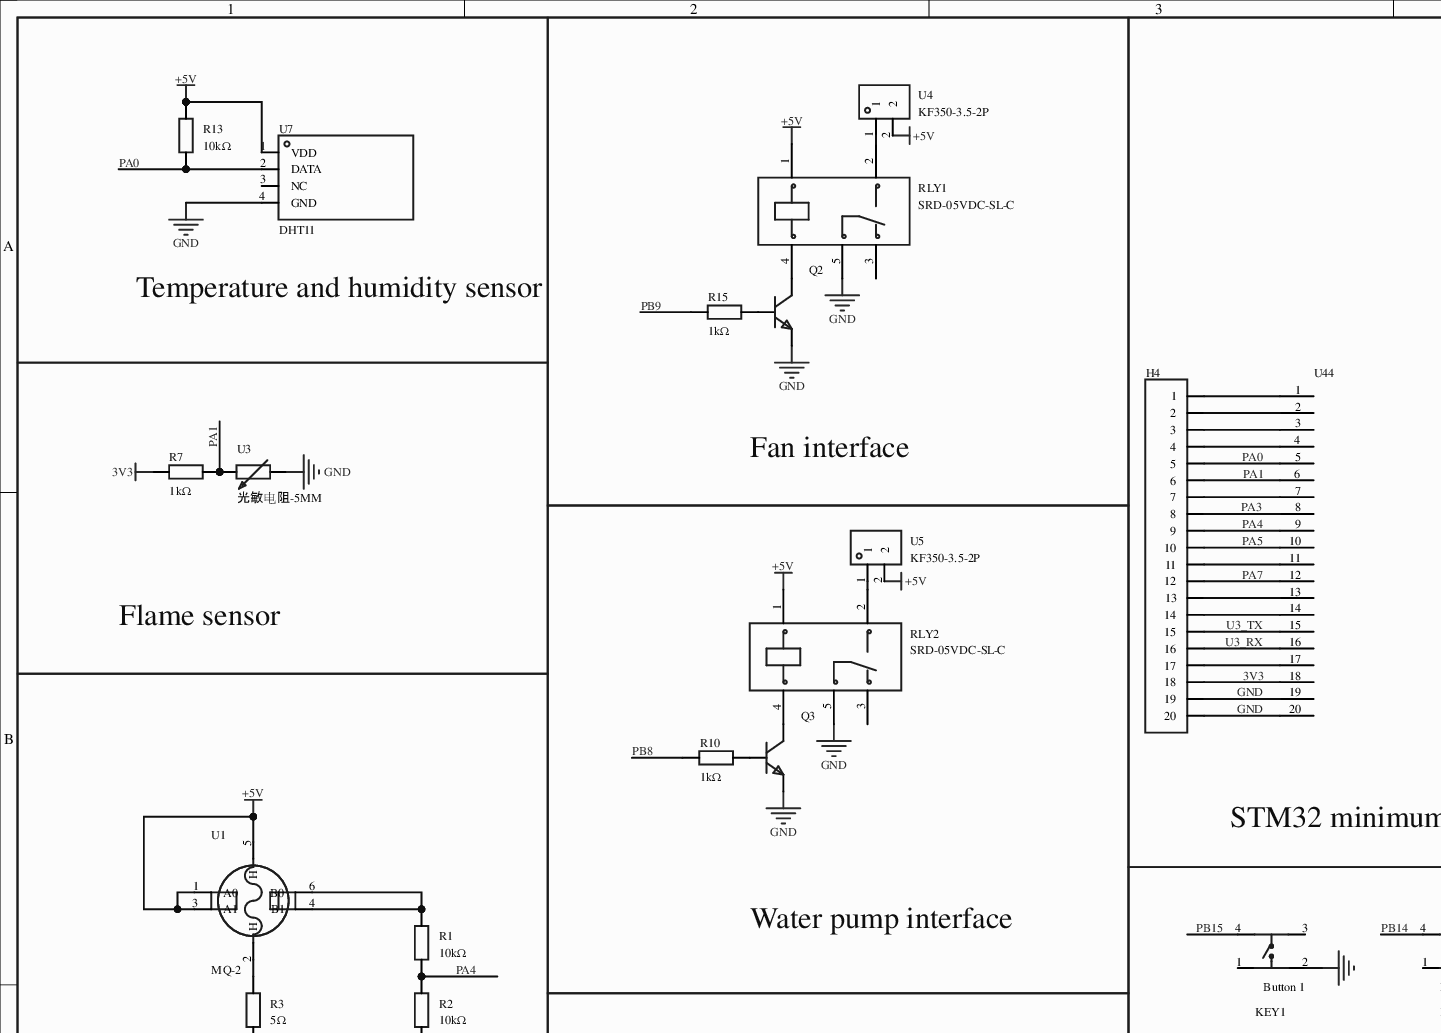
[diagram p0: MISC62290-3.schdoc, top left]
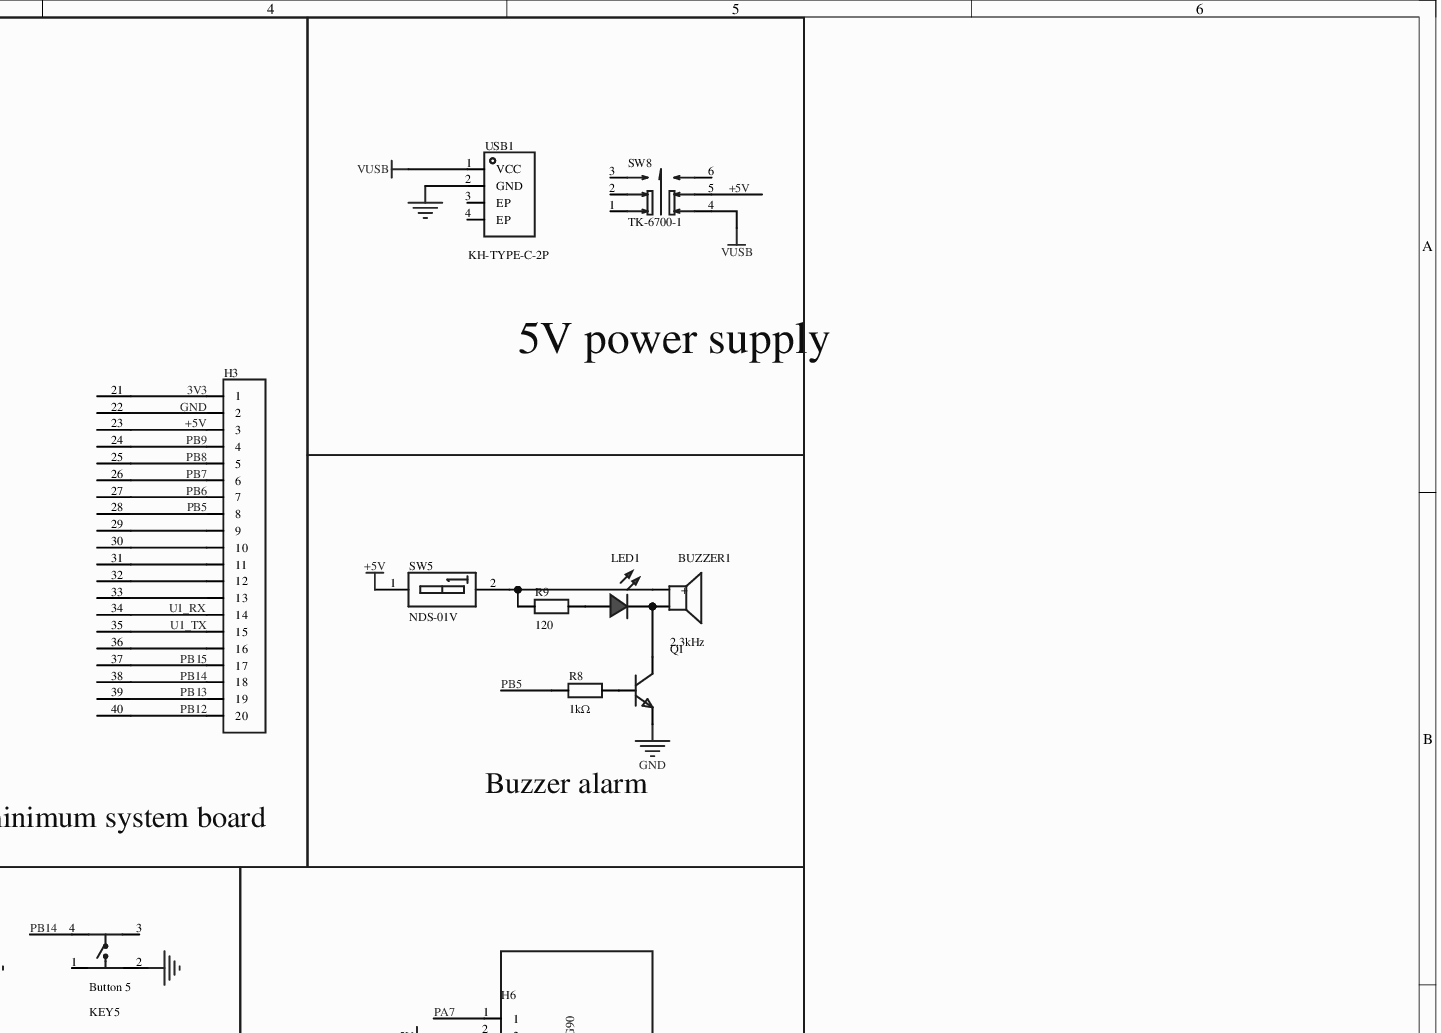
[diagram p1: MISC62290-3.schdoc, top right]
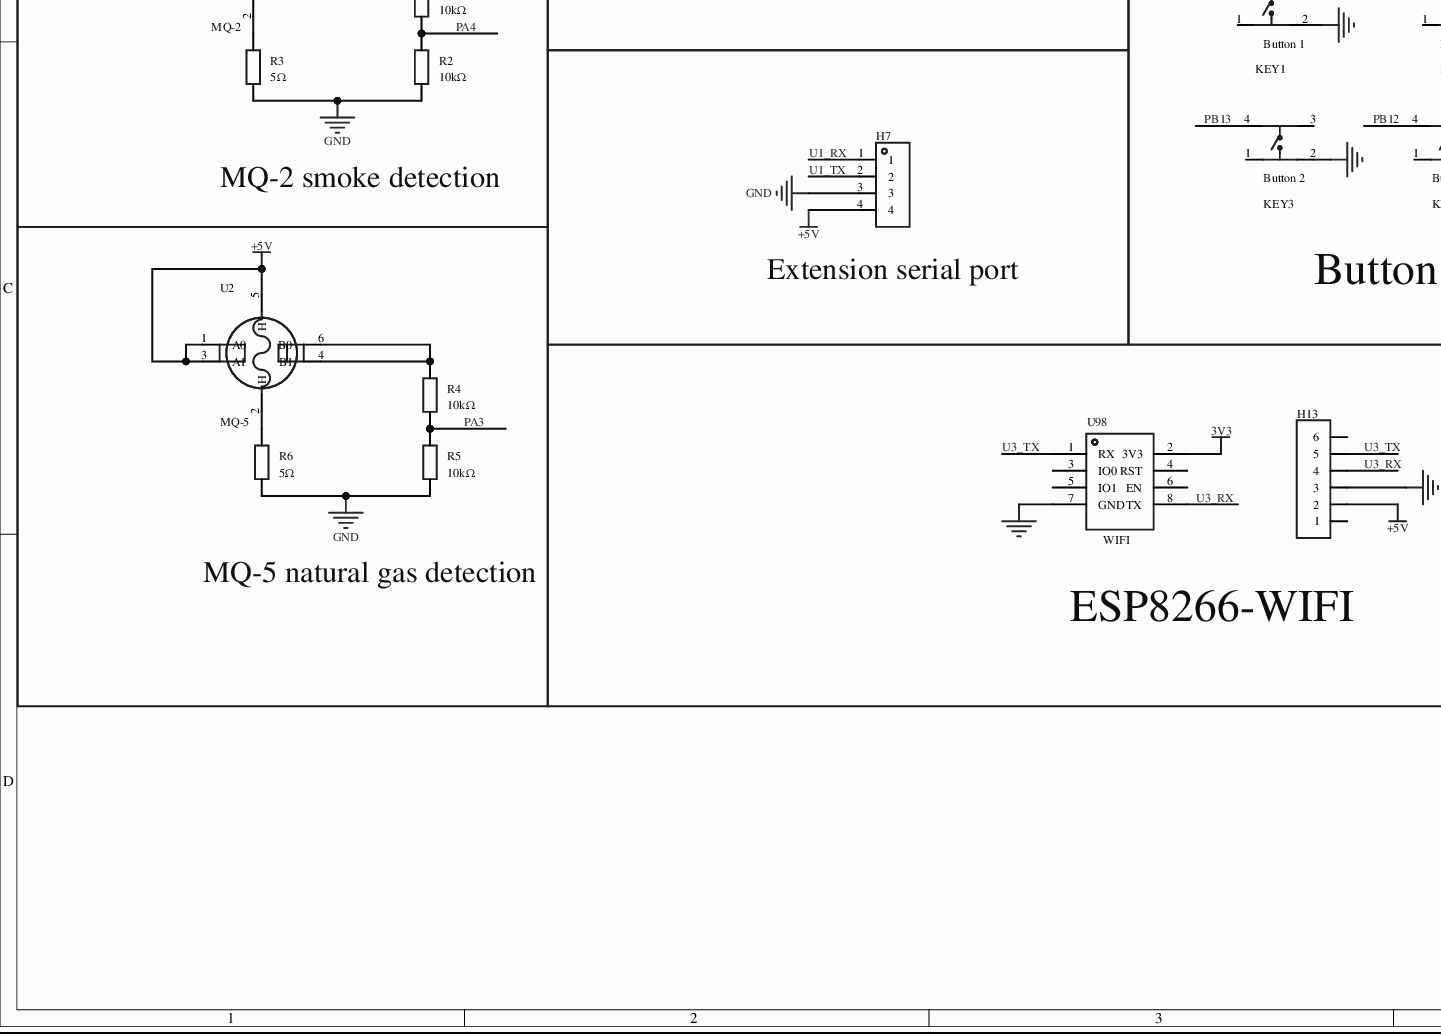
[diagram p2: MISC62290-3.schdoc, bottom left]
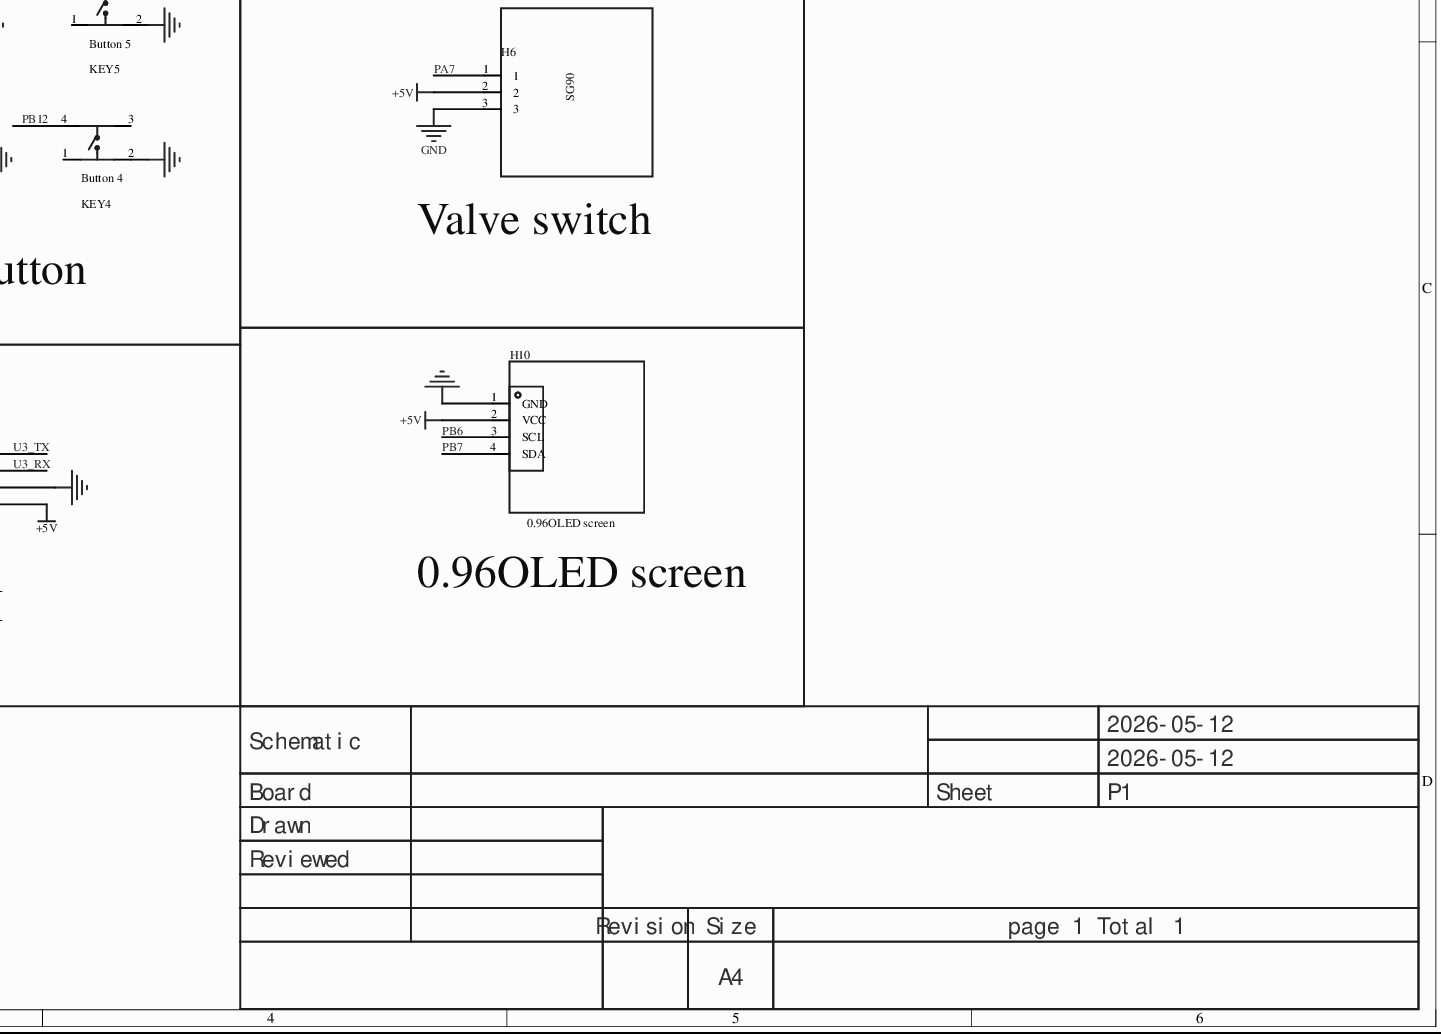
[diagram p3: MISC62290-3.schdoc, bottom right]
# Altium project MISC62290-2.PrjPcb
1 sheet, 40 parts. Net scope: global (net labels, ports and power ports of the same name join across sheets).
Board file: MISC62290.pcbdoc

## Sheet MISC62290-3.schdoc
size 420 x 297 mm; Version: V1.0; @Project Name: MISC62290; @Update Date: 2026-05-12; @Create Date: 2026-05-12; @Board Name: MISC62290; @Create Time: 10:51:37; @Page Count: 1; @Page No: 1; @Schematic Name: MISC62290; @Update Time: 10:51:37; Size: A4

### Parts
BUZZER1  2.3kHz  [BUZ-TH_BD12.0-P7.60-D0.6-FD]
H3  (no value)  [HDR-TH_20P-P2.54-V-F]
H4  (no value)  [HDR-TH_20P-P2.54-V-F]
H6  (no value)  [HDR-TH_3P-P2.54-V-F]
H7  (no value)  [HDR-TH_4P-P2.54-V-F]
H10  2.54-1*4P female  [HDR-TH_4P-P2.54-V-F]  (value not drawn)
H13  (no value)  [HDR-TH_6P-P2.54-V-M-1]
KEY1  Button 1  [KEY-TH_4P-L6.0-W6.0-P4.50-LS7.5]
KEY3  Button 2  [KEY-TH_4P-L6.0-W6.0-P4.50-LS7.5]
KEY4  Button 4  [KEY-TH_4P-L6.0-W6.0-P4.50-LS7.5]
KEY5  Button 5  [KEY-TH_4P-L6.0-W6.0-P4.50-LS7.5]
LED1  (no value)  [LED_TH-3mm]
Q1  (no value)  [S8050_TO_92]
Q2  (no value)  [S8050_TO_92]
Q3  (no value)  [S8050_TO_92]
R1  10kΩ  [Res_1/4W]
R2  10kΩ  [Res_1/4W]
R3  5Ω  [Res_1/4W]
R4  10kΩ  [Res_1/4W]
R5  10kΩ  [Res_1/4W]
R6  5Ω  [Res_1/4W]
R7  1kΩ  [Res_1/4W]
R8  1kΩ  [Res_1/4W]
R9  120  [Res_1/4W]
R10  1kΩ  [Res_1/4W]
R13  10kΩ  [Res_1/4W]
R15  1kΩ  [Res_1/4W]
RLY1  SRD-05VDC-SL-C  [RELAY-TH_SRD-XXVDC-XL-C]
RLY2  SRD-05VDC-SL-C  [RELAY-TH_SRD-XXVDC-XL-C]
SW5  NDS-01V  [SW-TH_2P-L3.9-W9.9-P2.54-LS7.6]
SW8  TK-6700-1  [SW-TH_TK-6700-1]
U1  MQ-2  [SENSOR-TH_MQ-2]
U2  MQ-5  [SENSOR-TH_MQ-2]
U3  光敏电阻-5MM  [RES-TH_L4.9-W4.3-P3.4]
U4  KF350-3.5-2P  [CONN-TH_P3.50_KF350-3.5-2P]
U5  KF350-3.5-2P  [CONN-TH_P3.50_KF350-3.5-2P]
U7  DHT11  [SENSOR-TH_DHT11]
U44  (no value)  [STM32最小系统板]
U98  (no value)  [WiFi封装]
USB1  KH-TYPE-C-2P  [USB-SMD_KH-TYPE-C-2P]

### Blocks framed on the sheet
Temperature and humidity sensor: R13 U7
Fan interface: Q2 R15 RLY1 U4
STM32 minimum system board: H3 H4 U44
5V power supply: SW8 USB1
Flame sensor: R7 U3
Buzzer alarm: BUZZER1 LED1 Q1 R8 R9 SW5
Water pump interface: Q3 R10 RLY2 U5
MQ-2 smoke detection: R1-R3 U1
Button: KEY1 KEY3-KEY5
Valve switch: H6
Extension serial port: H7
MQ-5 natural gas detection: R4-R6 U2
ESP8266-WIFI: H13 U98
0.96OLED screen: H10

### Nets
3V3: H3.1 H4.18 R7.1 U44.18 U44.21 U98.2(3V3)
+5V: H3.3 H6.2 H7.4 H10.2(VCC) H13.2 R13.2 RLY1.1 RLY2.1 SW5.1(A1) SW8.5 U1.1(A0) U1.3(A1) U1.5(H) U2.1(A0) U2.3(A1) U2.5(H) U4.2 U5.2 U7.1(VDD) U44.23
GND: H3.2 H4.19 H4.20 H6.3 H7.3 H10.1(GND) H13.3 KEY1.2 KEY3.2 KEY4.2 KEY5.2 Q1.1(E) Q2.1(E) Q3.1(E) R2.1 R3.1 R5.1 R6.1 RLY1.5 RLY2.5 U3.1 U7.4(GND) U44.19 U44.20 U44.22 U98.7(GND) USB1.2(GND)
VUSB: SW8.4 USB1.1(VCC)
PA0: H4.5 R13.1 U7.2(DATA) U44.5
PA1: H4.6 R7.2 U3.2 U44.6
PA3: H4.8 R4.1 R5.2 U44.8
PA4: H4.9 R1.1 R2.2 U44.9
PA5: H4.10 U44.10
PA7: H4.12 H6.1 U44.12
PB5: H3.8 R8.1 U44.28
PB6: H3.7 H10.3(SCL) U44.27
PB7: H3.6 H10.4(SDA) U44.26
PB8: H3.5 R10.1 U44.25
PB9: H3.4 R15.1 U44.24
PB12: H3.20 KEY4.4 U44.40
PB13: H3.19 KEY3.4 U44.39
PB14: H3.18 KEY5.4 U44.38
PB15: H3.17 KEY1.4 U44.37
U1_RX: H3.14 H7.1 U44.34
U1_TX: H3.15 H7.2 U44.35
U3_RX: H4.16 H13.4 U44.16 U98.8(TX)
U3_TX: H4.15 H13.5 U44.15 U98.1(RX)
NetBUZZER1_1: BUZZER1.1(+) R9.1 SW5.2(A2)
NetBUZZER1_2: BUZZER1.2 LED1.2(A) Q1.3(C)
NetH3_9: H3.9 U44.29
NetH3_10: H3.10 U44.30
NetH3_11: H3.11 U44.31
NetH3_12: H3.12 U44.32
NetH3_13: H3.13 U44.33
NetH3_16: H3.16 U44.36
NetH4_1: H4.1 U44.1
NetH4_2: H4.2 U44.2
NetH4_3: H4.3 U44.3
NetH4_4: H4.4 U44.4
NetH4_7: H4.7 U44.7
NetH4_11: H4.11 U44.11
NetH4_13: H4.13 U44.13
NetH4_14: H4.14 U44.14
NetH4_17: H4.17 U44.17
NetLED1_1: LED1.1(C) R9.2
NetQ1_2: Q1.2(B) R8.2
NetQ2_2: Q2.2(B) R15.2
NetQ2_3: Q2.3(C) RLY1.4
NetQ3_2: Q3.2(B) R10.2
NetQ3_3: Q3.3(C) RLY2.4
NetR1_2: R1.2 U1.4(B1) U1.6(B0)
NetR3_2: R3.2 U1.2(H)
NetR4_2: R4.2 U2.4(B1) U2.6(B0)
NetR6_2: R6.2 U2.2(H)
NetRLY1_2: RLY1.2 U4.1
NetRLY2_2: RLY2.2 U5.1

Not connected (* = marked no-connect by the designer): H13 1 6; KEY1 1 3*; KEY3 1 3*; KEY4 1 3*; KEY5 1 3*; RLY1 3; RLY2 3; SW8 1* 2* 3* 6*; U7 3(NC); U98 3(IO0) 4(RST) 5(IO1) 6(EN); USB1 3(EP) 4(EP)

### Notes on the sheet
- 2026-05-12
- Schematic
- Board
- Sheet
- P1
- Drawn
- Reviewed
- Revision
- Size
- A4
- page 1 Total 1

### Library data of the parts
BUZZER1 = TMB12A05_C96093: Drive method: active (built-in driver circuit); Construction type: electromagnetic; Rated voltage: 5V; Frequency: 2.3kHz; Sound pressure (SPL): 85dB@5V,10cm;; Manufacturer: 华能; 3D Model: 16ab50e14c5b4f2c986c135bdba60e37; 3D Model Transform: 472.44,472.176,0,90,0,0,-0.787,0,-177.165; Oscillator Circuit: Active (built-in driver); Operating Voltage: 4V~8V; AddInBom: yes; ModelName: BUZ-TH_D12.0-H9.5-P7.60; Symbol: TMB12A05; Device: TMB12A05_C96093; LCSC Part Name: TMB12A05; Supplier Part: C96093; Manufacturer Part: TMB12A05; Supplier Footprint: 插件,D=12mm; JLCPCB Part Class: Extended Part; Datasheet: https://atta.szlcsc.com/upload/public/pdf/source/20170522/1495448324811.pdf; Supplier: LCSC; Technology Type: Electromagnetic; Rated Voltage: 5V; Value: 2.3kHz; Sound Pressure Level (SPL): 85dB@5V,10cm; Diameter (φD): 12mm; Height: 9.8mm; ConvertToPcb: yes; FootprintName: BUZ-TH_BD12.0-P7.60-D0.6-FD
H3 H4 = HDR-F_2.54_1x20P: ConvertToPcb: yes; ModelId: db7015f7ad9d48b8a3b1188db02e34290819f05c4eef4c71ace90d822a990e87; ModelName: HDR-F-2.54_1x20; ModelTransform: 1999.996,100,0,0,0,0,0,0,-118.11; Symbol: HDR-F_2.54_1x20P; Device: HDR-F_2.54_1x20P; AddInBom: yes; SupplierPart: C50984; Supplier Footprint: 插件; FootprintName: HDR-TH_20P-P2.54-V-F
H6 = HDR-F_2.54_1x3P: Symbol: PM254V-11-03-H85_1; 3D Model: f3b3cc5aae9641bf9e56fc160cef875b; 3D Model Transform: 299.9994,100,0,0,0,0,0,0,-118.11; ConvertToPcb: yes; ModelName: HDR2.54-F-LI-1X3P; Device: HDR-F_2.54_1x3P; Supplier Part: C541850; Supplier Footprint: 插件; AddInBom: yes; FootprintName: HDR-TH_3P-P2.54-V-F
H7 = HDR-F_2.54_1x4P: Symbol: 2.54-1*4P female; ConvertToPcb: yes; ModelId: d187812051054f85879fcaa51a310d8e0819f05c4eef4c71ace90d822a990e87; ModelTransform: 419.6842,98.464,0,0,0,0,0,0,-118.11; Device: HDR-F_2.54_1x4P; AddInBom: yes; SupplierPart: C2718488; Supplier Footprint: 插件; FootprintName: HDR-TH_4P-P2.54-V-F; ModelName: HDR-TH_4P-P2.54-V-F
H10 = 0.96OLED屏幕: Socket structure: 1x4P; Pitch: 2.54mm; Row spacing: -; Round/square hole: square hole; Mounting type: through-hole; Rows: single row; Total positions: 4P; Rated current: 3A; Rated voltage: -; Socket direction: top; Plastic height: -; Contact material: bronze; Contact plating: -; Operating temperature range: -40℃~+105℃; Soldering temperature (max): -;; Manufacturer: BOOMELE(博穆精密); Manufacturer Part: 2.54-1*4P母; Symbol: 0.96OLED screen; 3D Model: 57daaad411c24bd7bd5d06edf5c4d16b; 3D Model Transform: 415.7472,98.425,0,0,0,0,0,0,-118.11; AddInBom: yes; ModelName: HDR-TH_4P-P2.54-F-LI-1X4P; Device: 0.96OLED screen; Supplier: LCSC; Supplier Part: C2718488; JLCPCB Part Class: Extension library; LCSC Part Name: 间距:2.54mm 1x4P 直插; Supplier Footprint: 插件,P=2.54mm; Datasheet: https://atta.szlcsc.com/upload/public/pdf/source/20210301/C2718488_F4427B881E42CAA8DDB0B1C12B3A522C.pdf; Holes Structure: 1x4P; Row Spacing: -; Circular Hole / Square Hole: Square hole; Mounting Type: Through-hole; Number of Rows: Single row; Number of Holes: 4P; Current Rating (Max): 3A; Voltage Rating (Max): -; Holes Direction: Top; Insulation Height: -; Contact Material: Bronze; Contact Plating: -; Operating Temperature Range: -40℃~+105℃; Soldering Temperature(Max): -; ConvertToPcb: yes; FootprintName: HDR-TH_4P-P2.54-V-F
H13 = HDR-M_2.54_1x6P: Symbol: Header-Male-2.54_1x6; 3D Model: 60739dffc9b04830a286435b0fefbd4a; 3D Model Transform: 599.999,100,0,0,0,0,0,0,-118.11; ConvertToPcb: yes; ModelName: HDR2.54-M-LI-1X6P; Device: HDR-M_2.54_1x6P; Supplier Part: C37208; Supplier Footprint: 插件; AddInBom: yes; FootprintName: HDR-TH_6P-P2.54-V-M-1
KEY1 = 按键开关6*6*8: Circuit structure: SPST; Contact rated current: -; Button head type: Round Button; Button actuation direction: Top Actuated;; Manufacturer Part: 按键1; Symbol: button6*6*8; Device: Tact switch 6*6*8; 3D Model: 84d39232fe0a426fa95ea2653754a6e5; 3D Model Transform: 306.868,236.22,0,0,0,0,0,0,-118.11; AddInBom: yes; ModelName: KEY-TH_4P-L6.0-W6.0-H4.5-LS6.5-P4.5; LCSC Part Name: 按键开关6*6*8   直插; Supplier Part: C59982; Supplier Footprint: Through Hole; JLCPCB Part Class: Extension library; Datasheet: https://atta.szlcsc.com/upload/public/pdf/source/20151126/1457707591845.pdf; Supplier: LCSC; ConvertToPcb: yes; FootprintName: KEY-TH_4P-L6.0-W6.0-P4.50-LS7.5
KEY3 = 按键开关6*6*8: Circuit structure: SPST; Contact rated current: -; Button head type: Round Button; Button actuation direction: Top Actuated;; Manufacturer Part: 按键2; Symbol: button6*6*8; Device: Tact switch 6*6*8; 3D Model: 84d39232fe0a426fa95ea2653754a6e5; 3D Model Transform: 306.868,236.22,0,0,0,0,0,0,-118.11; AddInBom: yes; ModelName: KEY-TH_4P-L6.0-W6.0-H4.5-LS6.5-P4.5; LCSC Part Name: 按键开关6*6*8   直插; Supplier Part: C59982; Supplier Footprint: Through Hole; JLCPCB Part Class: Extension library; Datasheet: https://atta.szlcsc.com/upload/public/pdf/source/20151126/1457707591845.pdf; Supplier: LCSC; ConvertToPcb: yes; FootprintName: KEY-TH_4P-L6.0-W6.0-P4.50-LS7.5
KEY4 = 按键开关6*6*8: Circuit structure: SPST; Contact rated current: -; Button head type: Round Button; Button actuation direction: Top Actuated;; Manufacturer Part: 按键4; Symbol: button6*6*8; Device: Tact switch 6*6*8; 3D Model: 84d39232fe0a426fa95ea2653754a6e5; 3D Model Transform: 306.868,236.22,0,0,0,0,0,0,-118.11; AddInBom: yes; ModelName: KEY-TH_4P-L6.0-W6.0-H4.5-LS6.5-P4.5; LCSC Part Name: 按键开关6*6*8   直插; Supplier Part: C59982; Supplier Footprint: Through Hole; JLCPCB Part Class: Extension library; Datasheet: https://atta.szlcsc.com/upload/public/pdf/source/20151126/1457707591845.pdf; Supplier: LCSC; ConvertToPcb: yes; FootprintName: KEY-TH_4P-L6.0-W6.0-P4.50-LS7.5
KEY5 = 按键开关6*6*8: Circuit structure: SPST; Contact rated current: -; Button head type: Round Button; Button actuation direction: Top Actuated;; Manufacturer Part: 按键5; Symbol: button6*6*8; Device: Tact switch 6*6*8; 3D Model: 84d39232fe0a426fa95ea2653754a6e5; 3D Model Transform: 306.868,236.22,0,0,0,0,0,0,-118.11; AddInBom: yes; ModelName: KEY-TH_4P-L6.0-W6.0-H4.5-LS6.5-P4.5; LCSC Part Name: 按键开关6*6*8   直插; Supplier Part: C59982; Supplier Footprint: Through Hole; JLCPCB Part Class: Extension library; Datasheet: https://atta.szlcsc.com/upload/public/pdf/source/20151126/1457707591845.pdf; Supplier: LCSC; ConvertToPcb: yes; FootprintName: KEY-TH_4P-L6.0-W6.0-P4.50-LS7.5
LED1 = LED_TH-R_3mm: ConvertToPcb: yes; ModelId: a497c992633541038a38947cdc58012f0819f05c4eef4c71ace90d822a990e87; ModelName: LED-TH-3mm_R; ModelTransform: 141.274,153.327,0,0,0,0,-5.984,0,-137.795; Symbol: LED_TH-R; Device: LED_TH-R_3mm; AddInBom: yes; FootprintName: LED_TH-3mm; Supplier Footprint: 插件
Q1-Q3 = S8050_TO_NPN: 3D Model: aafe8e06f2154e7c93506efd0d6632dd; 3D Model Transform: 180.78,141.44,417.3,0,0,0,0,0,-200; ConvertToPcb: yes; ModelName: TO-92-3_L4.9-W3.7-P1.27-L; Symbol: S8050_TO_NPN; Device: S8050_TO_NPN; Supplier Footprint: TO-92; AddInBom: yes; FootprintName: S8050_TO_92
R1-R3 R10 R13 R15 = Res_AXIAL-1/8W: Symbol: Resistor; 3D Model: b2b5ae7ae4c642178fe0039925c86a3f0819f05c4eef4c71ace90d822a990e87; 3D Model Transform: 282.86,66.88,253.09,0,0,0,0,0,-191; ConvertToPcb: yes; ModelName: RES-TH_BD1.8-L3.2-P7.20-D0.4; Device: Res_AXIAL-1/8W; Supplier Footprint: 轴向引线; AddInBom: yes; FootprintName: Res_1/4W
  R1 R2 R13: Value: 10kΩ
  R3: Value: 5Ω
  R10 R15: Value: 1kΩ
R4-R6 = Res_AXIAL-1/8W: Symbol: Resistor; ConvertToPcb: yes; ModelId: b2b5ae7ae4c642178fe0039925c86a3f0819f05c4eef4c71ace90d822a990e87; ModelName: RES-TH_BD1.8-L3.2-P7.20-D0.4; ModelTransform: 282.86,66.88,253.09,0,0,0,0,0,-191; Device: Res_AXIAL-1/8W; AddInBom: yes; Supplier Footprint: 轴向引线; FootprintName: Res_1/4W
  R4 R5: Value: 10kΩ
  R6: Value: 5Ω
R7 = Res_AXIAL-1/4W: Symbol: Resistor; 3D Model: 463263665006444ab7a47bd11b0cf9560819f05c4eef4c71ace90d822a990e87; 3D Model Transform: 427.165,94.32816,0,0,0,0,0,0,-196.85; AddInBom: yes; ModelName: RES-TH_BD2.4-L6.3-P10.30-D0.6; Device: Res_AXIAL-1/4W; Supplier Footprint: 轴向引线; Value: 1kΩ; ConvertToPcb: yes; FootprintName: Res_1/4W
R8 R9 = Res_AXIAL-1/4W: Symbol: Resistor; 3D Model: 463263665006444ab7a47bd11b0cf956; 3D Model Transform: 427.165,94.32816,0,0,0,0,0,0,-196.85; AddInBom: yes; ModelName: RES-TH_BD2.4-L6.3-P10.30-D0.6; Device: Res_AXIAL-1/4W; Supplier Footprint: 轴向引线; ConvertToPcb: yes; FootprintName: Res_1/4W
  R8: Value: 1kΩ
  R9: Value: 120
RLY1 RLY2 = SRD-05VDC-SL-C: Coil voltage: 5V; Contact form: 1C changeover (SPDT); Contact capacity (resistive load): -; Max switching voltage: 250V@AC; Max switching current: 15A;; Manufacturer: 松乐; AddInBom: yes; ModelId: d0eda9b8bf8746d18ae810ab88dc78e70819f05c4eef4c71ace90d822a990e87; ModelName: RELAY-TH_L19.2-W15.6-H15.8; ModelTransform: 755.904,622.4397,0,0,0,0,34.882,0,-118.11; Coil Rated Power: 360mW; Coil Type: Non-polar, single coil; Coil Resistance: 70Ω; Contact Resistance: 100mΩ; Operate Time: 10ms; Symbol: SRD-05VDC-SL-C; Device: SRD-05VDC-SL-C; LCSC Part Name: 蓝色 单组转换型继电器; SupplierPart: C35449; ManufacturerPart: SRD-05VDC-SL-C; Supplier Footprint: 插件,19.2x15.6mm; JLCPCB Part Class: Extended Part; Datasheet: https://item.szlcsc.com/datasheet/SRD-05VDC-SL-C/36422.html; Supplier: LCSC; ConvertToPcb: yes; FootprintName: RELAY-TH_SRD-XXVDC-XL-C; Coil Voltage: 5V; Contact Form: 1C changeover (SPDT); Number of Pins: 5; Contact Rating: -; Switching Voltage(Max): 250V@AC; Switching Current(Max): 15A; Release Time: 10ms
SW5 = NDS-01V_C501305: Tall lever, forward action; 3D Model: a6fe51954c31461ebc9e88beb6e51f3d0819f05c4eef4c71ace90d822a990e87; 3D Model Transform: 161.417,389.763,0,270,0,0,0,0,-125.984; AddInBom: yes; ModelName: SW-TH_L4.0-W9.9-H5.4-P2.54-B; Symbol: NDS-01V; Device: NDS-01V_C501305; LCSC Part Name: 拨码开关; Supplier Part: C501305; Manufacturer Part: NDS-01V; Supplier Footprint: DIP; JLCPCB Part Class: Extended Part; Supplier: LCSC; ConvertToPcb: yes; FootprintName: SW-TH_2P-L3.9-W9.9-P2.54-LS7.6
SW8 = TK-6700-1: Manufacturer: Yuandi(元迪); 3D Model: 1dccfbf2ceb24a728093c1f6ee61932a; 3D Model Transform: 275.59,275.59,0,90,0,0,0,0,-137.795; AddInBom: yes; Symbol: TK-6700-1; Device: TK-6700-1; LCSC Part Name: 自锁开关7*7*12.7有声有锁高导高柄插件双排6P按键开关带锁DIP六脚; Supplier Part: C528782; Manufacturer Part: TK-6700-1; Supplier Footprint: 插件; JLCPCB Part Class: Extended Part; Datasheet: https://atta.szlcsc.com/upload/public/pdf/source/20200831/C528782_58F076EBF84BD8A9E2DE38DB1C0986D4.pdf; Supplier: LCSC; ConvertToPcb: yes; FootprintName: SW-TH_TK-6700-1; ModelName: SW-TH_TK-6700-1
U1 U2 = MQ-2: Manufacturer: Winsen(炜盛); 3D Model: a4c1c1cdd77042ea8ff9a8560a5de51a0819f05c4eef4c71ace90d822a990e87; 3D Model Transform: 747.59323,747.81158,0,0,0,0,0,0,-393.701; AddInBom: yes; Symbol: MQ-2; Device: MQ-2; LCSC Part Name: 可燃气体传感器; Supplier Part: C99296; Supplier Footprint: 插件; JLCPCB Part Class: Extended Part; Datasheet: https://atta.szlcsc.com/upload/public/pdf/source/20180502/C99296_6F0BA5D7AA10C610B74ABFD8A5ECF346.pdf; Supplier: LCSC; ConvertToPcb: yes; FootprintName: SENSOR-TH_MQ-2; ModelName: SENSOR-TH_MQ-2
  U1: Manufacturer Part: MQ-2
  U2: Manufacturer Part: MQ-5
U3 = 光敏电阻-5MM: AddInBom: yes; ModelId: 8cda4899688949e78503a56fe341541c0819f05c4eef4c71ace90d822a990e87; ModelTransform: 169.291,200.6107,0,90,0,0,0,0,-196.85; Symbol: 光敏电阻-5MM; Device: 光敏电阻-5MM; LCSC Part Name: 光敏电阻-5MM; SupplierPart: C9900003115; ManufacturerPart: 光敏电阻-5MM; Supplier Footprint: RES-TH_4.3X4.9X3.37P; JLCPCB Part Class: Extended Part; Supplier: LCSC; ConvertToPcb: yes; FootprintName: RES-TH_L4.9-W4.3-P3.4; ModelName: RES-TH_L4.9-W4.3-P3.4
U4 U5 = KF350-3.5-2P: Structure: 1x2P; Pitch: 3.5mm; Color: green; Mounting: through-hole; Rated current: 10A; Rated voltage: 300V; Rows: 1; Wire gauge - AWG: 18~24; Wire gauge - mm²: 0.75; Pins per row: 2; Operating temperature range: -40℃~+105℃;; Manufacturer: KEFA(科发); AddInBom: yes; ModelId: b1d1e83e7d6a49aab33370f0163c64ca0819f05c4eef4c71ace90d822a990e87; ModelTransform: 314.96,271.653,0,0,0,0,0,1.968,-133.858; Wire Gauge - mm2: 0.75; Number of PINs Per Row: 2; Symbol: KF350-3.5-2P; Device: KF350-3.5-2P; LCSC Part Name: 3.5mm 1x2P 排数:1 每排P数:2 直插; SupplierPart: C474892; ManufacturerPart: KF350-3.5-2P; Supplier Footprint: 插件,P=3.5mm; JLCPCB Part Class: Extended Part; Datasheet: https://atta.szlcsc.com/upload/public/pdf/source/20230317/986DB56DD49619EA586AA8816AA9D164.pdf; Supplier: LCSC; ConvertToPcb: yes; FootprintName: CONN-TH_P3.50_KF350-3.5-2P; ModelName: CONN-TH_P3.50_KF350-3.5-2P; Color: Green; Mounting Style: Through-hole; Current Rating (Max): 10A; Voltage Rating (Max): 300V; Number of Pins: 2P; Number of Rows: 1; Wire Gauge - AWG: 18~24; Operating Temperature Range: -40℃~+105℃
U7 = DHT11: Temperature range: -20℃~+60℃; humidity range: 5%RH~95%RH; humidity accuracy: ±5%RH;; Manufacturer: 广州奥松; AddInBom: yes; ModelId: 6dde47d4d8bf4fa598dffcc067449c1d0819f05c4eef4c71ace90d822a990e87; ModelTransform: 236.25937,492.125,0,270,0,0,0,-11.811,-196.85; Voltage - Supply: 3.3V~5.5V; Current - Supply: 1mA; Temperature Tolerance: ±2℃; Symbol: DHT11; Device: DHT11; LCSC Part Name: 新款电容式数字温湿度传感器,老款已停产16.1x12.6x5.8mm DHT11  电容式传感器; SupplierPart: C117051; ManufacturerPart: DHT11; Supplier Footprint: SIP-4; JLCPCB Part Class: Extended Part; Datasheet: https://item.szlcsc.com/datasheet/DHT11/118309.html; Supplier: LCSC; ConvertToPcb: yes; FootprintName: SENSOR-TH_DHT11; ModelName: SENSOR-TH_DHT11; Temperature Range: -20℃~+60℃; Humidity: 5%RH~95%RH; Humidity Tolerance: ±5%RH
U44 = STM32最小系统板: Symbol: STM32 minimum system board; AddInBom: yes; Device: STM32 minimum system board; ConvertToPcb: yes; FootprintName: STM32 minimum system board
U98 = WiFi模块: Symbol: WiFi module; AddInBom: yes; Device: WiFi module; ConvertToPcb: yes; FootprintName: WiFi footprint
USB1 = KH-TYPE-C-2P: Connector type: Type-C; Standard: -; Male/female: -; Port count: -; Contact count: 2P; Mounting: -; Rated current - power: -; Contact material: -; Contact plating: -; Operating temperature range: -;; Manufacturer: kinghelm(金航标); 3D Model: 4464b34a7d0f48c2b8c2350e914c93f5; 3D Model Transform: 352.362,255.31449,0,0,0,0,0,-49.213,-98.425; Current Rating-Power: 3A; Voltage Rating: 20V; Connect-Disconnect Life: 5 thousand cycles; AddInBom: yes; Symbol: KH-TYPE-C-2P; Device: KH-TYPE-C-2P; LCSC Part Name: Type-C; Supplier Part: C2919656; Manufacturer Part: KH-TYPE-C-2P; Supplier Footprint: 插件; JLCPCB Part Class: Extended Part; Datasheet: https://atta.szlcsc.com/upload/public/pdf/source/20220707/620587A9E0589B27D96D3CEE595CBC98.pdf; Supplier: LCSC; Connector Type: Type-C; Gender: -; Number of Ports: -; Number of Contacts: 2P; Mounting Style: -; Current Rating - Power (Max): -; Contact Material: -; Contact Plating: -; Operating Temperature Range: -; Protocol Standard: -; Mounting Type: Right angle; Length: 6.43mm; Operating Temperature: -25℃~+85℃; ConvertToPcb: yes; FootprintName: USB-SMD_KH-TYPE-C-2P; ModelName: USB-SMD_KH-TYPE-C-2P